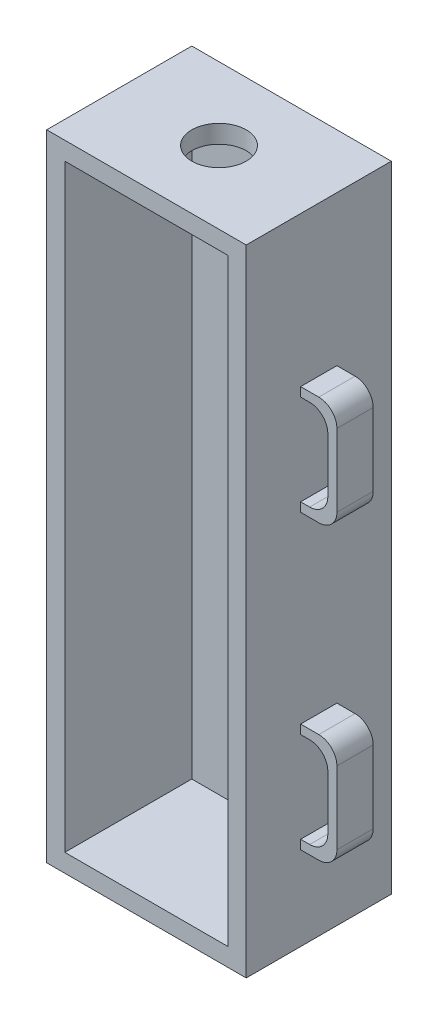
from build123d import *

# Parameters (mm, degrees)
SKETCH1_W            = 110
SKETCH1_H            = 350
BOSS_EXTRUDE1_DEPTH  = 80
SHELL1_T             = -10
SKETCH2_W            = 20
SKETCH2_H            = 60
BOSS_EXTRUDE2_DEPTH  = 20
SKETCH3_W            = 15
SKETCH3_H            = 50
CUT_EXTRUDE1_DEPTH   = 50
FILLET1_R            = 10
FILLET1_OF_MIRROR1_R = 10
SKETCH4_R            = 15
CUT_EXTRUDE2_DEPTH   = 50


with BuildPart() as part:
    # Sketch1 → Boss-Extrude1 (new body)
    with BuildSketch(Plane.XY):
        with Locations((-119, 670)):
            Rectangle(SKETCH1_W, SKETCH1_H)
    extrude(amount=BOSS_EXTRUDE1_DEPTH)

    # Shell1
    shell1_openings = [part.faces().sort_by_distance(p)[0] for p in [
        (-119, 670, 80),
    ]]
    offset(amount=SHELL1_T, openings=shell1_openings, kind=Kind.INTERSECTION)

    # Sketch2 → Boss-Extrude2 (add)
    with BuildSketch(Plane.ZY.offset(174)):
        with Locations((40, 732.363495956)):
            Rectangle(SKETCH2_W, SKETCH2_H)
        with Locations((40, 571.241967209)):
            Rectangle(SKETCH2_W, SKETCH2_H)
    boss_extrude2 = extrude(amount=BOSS_EXTRUDE2_DEPTH)

    # Sketch3 → Cut-Extrude1 (cut)
    with BuildSketch(Plane.XY.offset(50)):
        Polygon((-179, 596.241967209), (-174, 596.241967209), (-174, 546.241967209), (-179, 546.241967209), (-189, 546.241967209), (-189, 596.241967209), align=None)
        with Locations((-181.5, 732.363495956)):
            Rectangle(SKETCH3_W, SKETCH3_H)
    cut_extrude1 = extrude(amount=-CUT_EXTRUDE1_DEPTH, mode=Mode.SUBTRACT)

    # Fillet1
    fillet1_edges = [part.edges().sort_by_distance(p)[0] for p in [
        (-194, 702.363495956, 40),
        (-194, 762.363495956, 40),
        (-194, 541.241967209, 40),
        (-194, 601.241967209, 40),
        (-189, 546.241967209, 40),
        (-189, 596.241967209, 40),
        (-189, 707.363495956, 40),
        (-189, 757.363495956, 40),
    ]]
    fillet(fillet1_edges, radius=FILLET1_R)

    # Mirror1: Boss-Extrude2, Cut-Extrude1 across plane
    add(boss_extrude2.mirror(Plane(origin=(-119, 0, 0), x_dir=(0, 0, 1), z_dir=(1, 0, 0))))
    add(cut_extrude1.mirror(Plane(origin=(-119, 0, 0), x_dir=(0, 0, 1), z_dir=(1, 0, 0))), mode=Mode.SUBTRACT)

    # Fillet1 of Mirror1
    fillet1_of_mirror1_edges = [part.edges().sort_by_distance(p)[0] for p in [
        (-44, 702.363495956, 40),
        (-44, 762.363495956, 40),
        (-44, 541.241967209, 40),
        (-44, 601.241967209, 40),
        (-49, 546.241967209, 40),
        (-49, 596.241967209, 40),
        (-49, 707.363495956, 40),
        (-49, 757.363495956, 40),
    ]]
    fillet(fillet1_of_mirror1_edges, radius=FILLET1_OF_MIRROR1_R)

    # Sketch4 → Cut-Extrude2 (cut)
    with BuildSketch(Plane(origin=(0, 845, 0), x_dir=(1, 0, 0), z_dir=(0, 1, 0))):
        with Locations(Location((-119, -40, 0), (0, 0, 270))):
            Circle(SKETCH4_R)
    extrude(amount=-CUT_EXTRUDE2_DEPTH, mode=Mode.SUBTRACT)


solid = part.part
